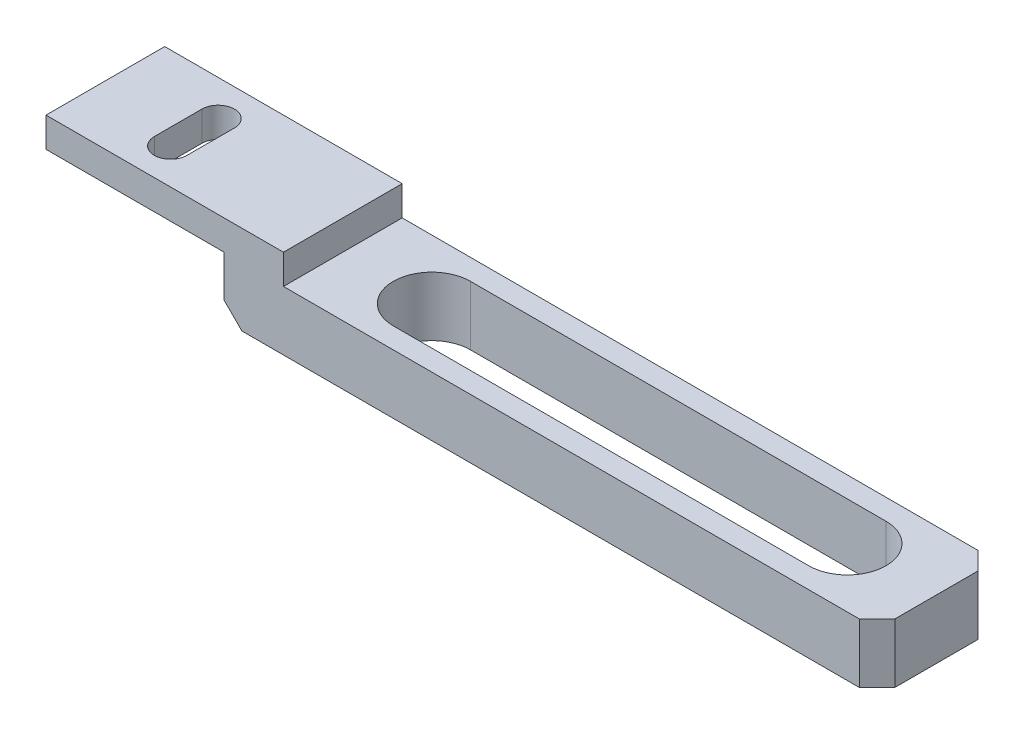
SolidWorks part; units mm, degrees
material "6061 合金"
ref_plane "前视基准面" through (0, 0, 0) normal (0, 0, 1) x (1, 0, 0)
ref_plane "上视基准面" through (0, 0, 0) normal (0, 1, 0) x (1, 0, 0)
ref_plane "右视基准面" through (0, 0, 0) normal (1, 0, 0) x (0, 0, -1)
sketch "草图2" plane through (0, 0, 0) normal (0, 0, 1) x (1, 0, 0)
  line L0 (0, 0) -> (140, 0)
  line L3 (140, 0) -> (140, -15)
  line L4 (140, -15) -> (30, -15)
  line L5 (30, -15) -> (30, -5)
  line L6 (30, -5) -> (0, -5)
  line L7 (0, -5) -> (0, 0)
  dimension "D1" = 5
  dimension "D2" = 30
  dimension "D5" = 110
  dimension "D6" = 15
extrude "凸台-拉伸1" add sketch "草图2" along normal mid plane 20
sketch "草图3" plane through (0, 0, 0) normal (0, 1, 0) x (1, 0, 0)
  line L0 (55, 0) -> (125, 0) construction
  line L1 (55, 6.5) -> (125, 6.5)
  line L2 (55, -6.5) -> (125, -6.5)
  line L4 (140, -10) -> (140, 10) construction
  arc A0 (55, 6.5) -> (55, -6.5) centre (55, 0) ccw
  arc A1 (125, -6.5) -> (125, 6.5) centre (125, 0) ccw
  point P3 (90, 0)
  dimension "D1" = 13
  dimension "D2" = 15
  dimension "D3" = 55
extrude "切除-拉伸1" cut sketch "草图3" against normal through all
sketch "草图4" plane through (0, 0, 0) normal (0, 1, 0) x (1, 0, 0)
  line L0 (15, 4) -> (15, -4) construction
  line L1 (17.75, 4) -> (17.75, -4)
  line L2 (12.25, 4) -> (12.25, -4)
  line L3 (0, -10) -> (0, 10) construction
  arc A0 (17.75, 4) -> (12.25, 4) centre (15, 4) ccw
  arc A1 (12.25, -4) -> (17.75, -4) centre (15, -4) ccw
  point P2 (15, 0)
  dimension "D1" = 5.5
  dimension "D2" = 15
  dimension "D3" = 8
extrude "切除-拉伸2" cut sketch "草图4" against normal through all
chamfer "倒角1" distance 3 angle 45 2 edges at (140, -7.5, -10) (140, -7.5, 10)
chamfer "倒角2" distance 3 angle 45 1 edges at (30, -15, 0)
sketch "草图5" plane through (0, 0, 10) normal (0, 0, 1) x (1, 0, 0)
  line L0 (30, -5) -> (30, -12) construction
  line L1 (140, 0) -> (40, 0)
  line L2 (140, 0) -> (140, -5)
  line L3 (140, -5) -> (40, -5)
  line L4 (40, 0) -> (40, -5)
  line L5 (33, -15) -> (137, -15) construction
  dimension "D1" = 10
  dimension "D2" = 10
extrude "切除-拉伸3" cut sketch "草图5" against normal through all
